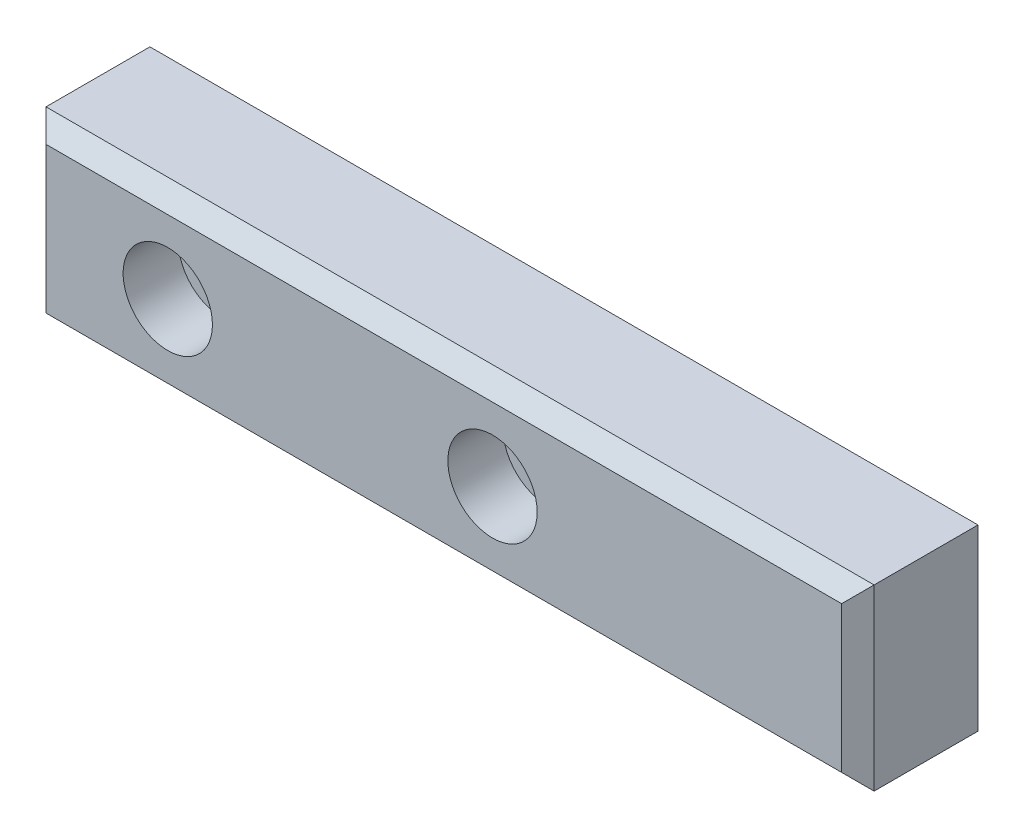
SolidWorks part; units mm, degrees
material "Aluminum Profile"
ref_plane "Front Plane" through (0, 0, 0) normal (0, 0, 1) x (1, 0, 0)
ref_plane "Top Plane" through (0, 0, 0) normal (0, 1, 0) x (1, 0, 0)
ref_plane "Right Plane" through (0, 0, 0) normal (1, 0, 0) x (0, 0, -1)
sketch "Sketch1" plane through (0, 0, 0) normal (0, 0, 1) x (1, 0, 0)
  line L1 (51, -11) -> (-51, -11)
  line L2 (51, -11) -> (51, 11)
  line L3 (51, 11) -> (-51, 11)
  line L4 (-51, -11) -> (-51, 11)
  line L5 (51, -11) -> (-51, 11) construction
  line L6 (51, 11) -> (-51, -11) construction
  point P0 (0, 0)
  dimension "D1" = 22
  dimension "D2" = 102
extrude "Boss-Extrude1" add sketch "Sketch1" along normal blind 15
hole_wizard "Hole size per socket head cap screw type1" positions "3DSketch1" profile "Sketch2" counterbore size "M6" standard "Gb" end condition through all
sketch3d "3DSketch1"
  line L0 (51, 11, 15) -> (-51, 11, 15) construction
  line L1 (-51, 11, 15) -> (-51, -11, 15) construction
  point P0 (-34, 0, 15)
  point P2 (6, 0, 15)
  dimension "D1" = 11
  dimension "D2" = 17
  dimension "D3" = 40
sketch "Sketch2" plane through (-34, 0, 15) normal (1, 0, 0) x (0, -1, 0)
  line L0 (0, 0) -> (0, 15)
  line L1 (0, 15) -> (3.3, 15)
  line L3 (3.3, 15) -> (3.3, 6.8)
  line L4 (3.3, 6.8) -> (5.5, 6.8)
  line L5 (5.5, 6.8) -> (5.5, 0)
  line L7 (5.5, 0) -> (0, 0)
  line L11 (0, -6.35) -> (0, 107.95) construction
  dimension "通孔孔直径" = 6.6
  dimension "通孔孔深度" = 15
  dimension "柱形沉头孔直径" = 11
  dimension "柱形沉头孔深度" = 6.8
chamfer "Chamfer1" distance 0.2 angle 45 4 edges at (-51, 0, 0) (0, -11, 0) (51, 0, 0) (0, 11, 0)
chamfer "Chamfer2" distance 2 angle 45 4 edges at (51, 0, 15) (0, -11, 15) (-51, 0, 15) (0, 11, 15)
